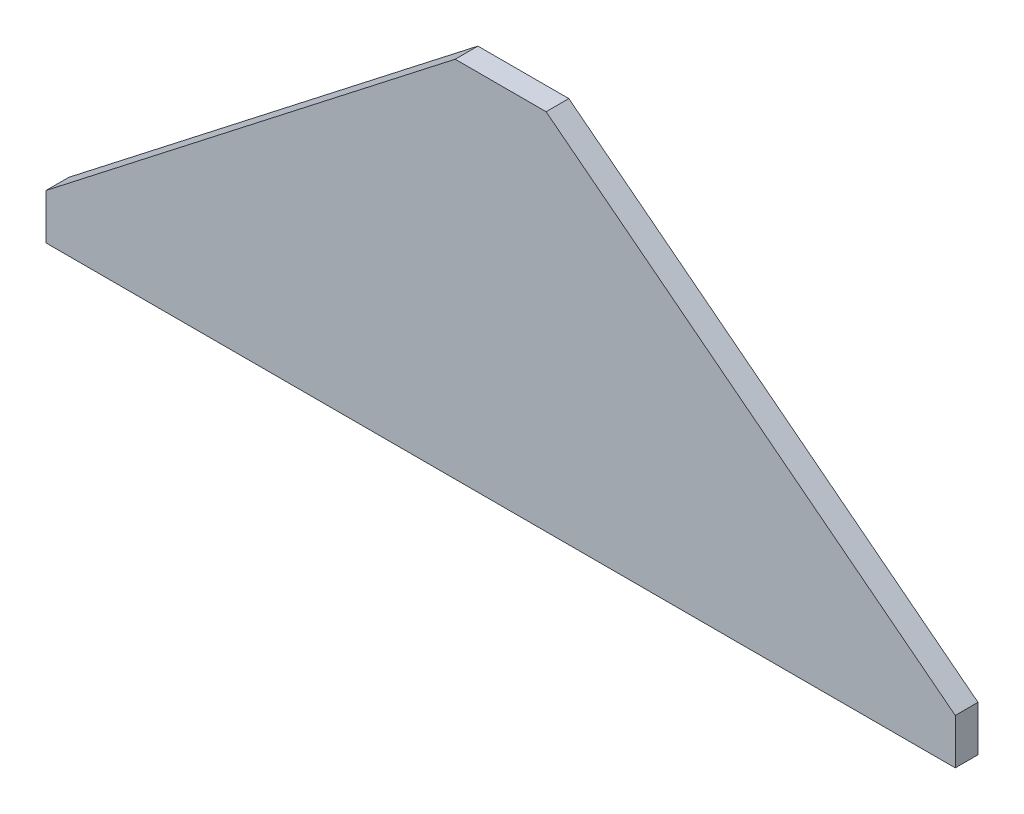
SolidWorks part; units mm, degrees
material "1023 碳钢板 (SS)"
ref_plane "前视基准面" through (0, 0, 0) normal (0, 0, 1) x (1, 0, 0)
ref_plane "上视基准面" through (0, 0, 0) normal (0, 1, 0) x (1, 0, 0)
ref_plane "右视基准面" through (0, 0, 0) normal (1, 0, 0) x (0, 0, -1)
sketch "草图1" plane through (0, 0, 0) normal (0, 0, 1) x (1, 0, 0)
  line L0 (-10, 20.2301) -> (-100, -49.7699)
  line L1 (-10, 20.2301) -> (10, 20.2301)
  line L2 (-100, -49.7699) -> (-100, -59.7699)
  line L3 (-100, -59.7699) -> (100, -59.7699)
  line L4 (100, -49.7699) -> (100, -59.7699)
  line L7 (10, 20.2301) -> (100, -49.7699)
  point P0 (0, 20.2301)
  point P2 (0, 0)
  point P4 (0, 0)
  dimension "D1" = 70
  dimension "D2" = 200
  dimension "D3" = 10
  dimension "D4" = 70
  dimension "D5" = 20
extrude "凸台-拉伸1" add sketch "草图1" along normal blind 5
